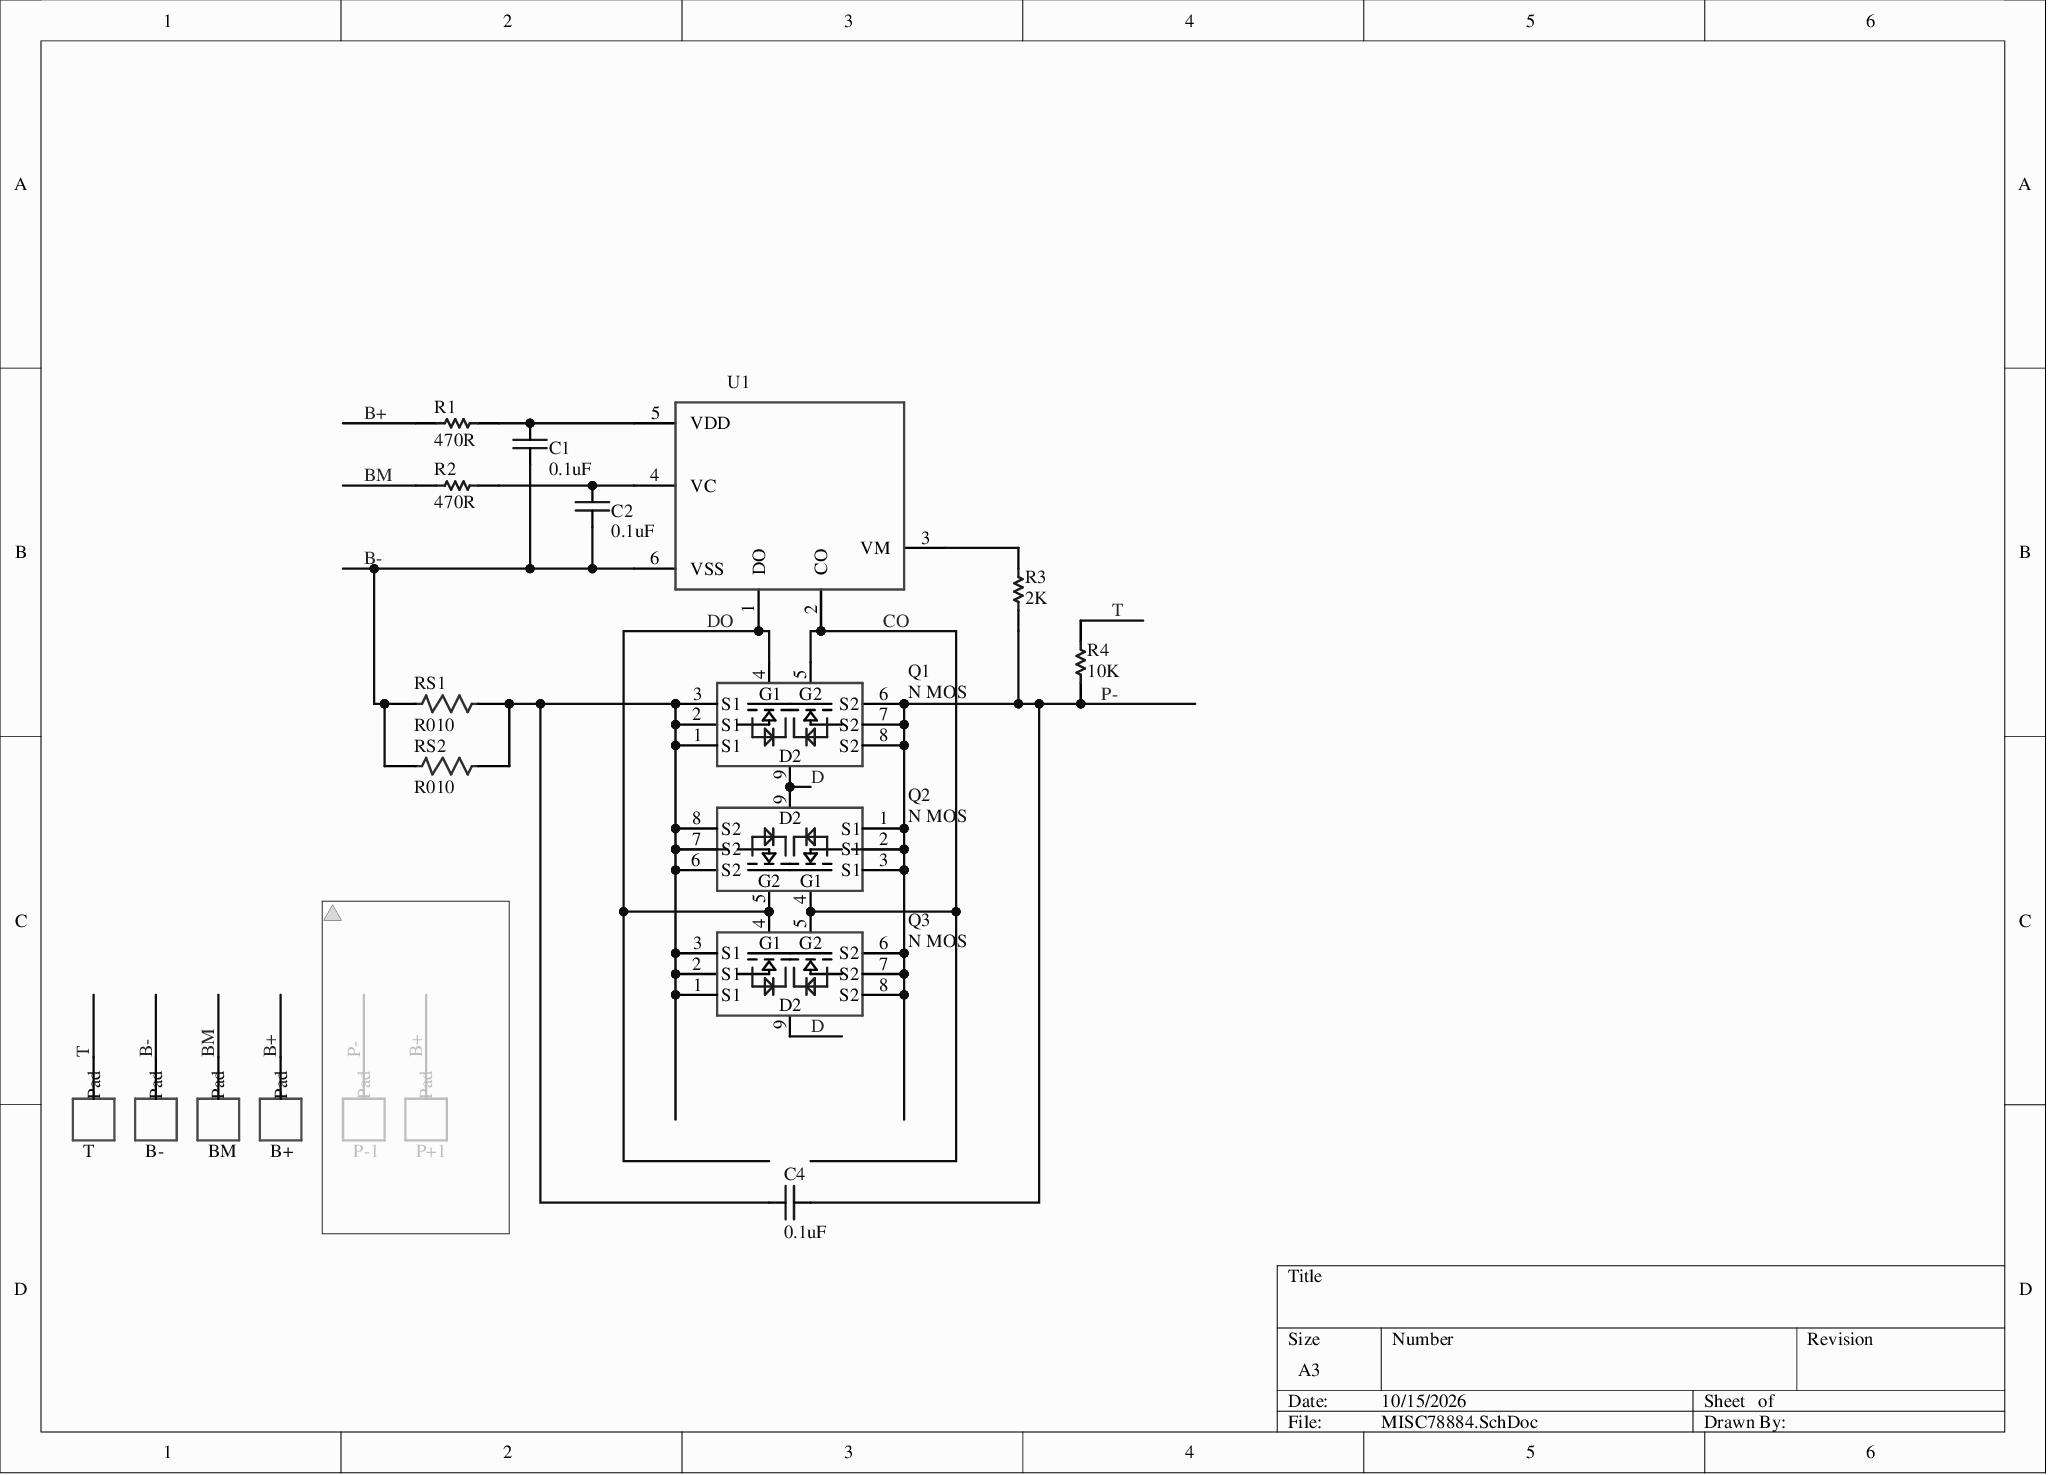
[diagram p0: MISC78884.SchDoc]
# Altium project MISC78884.PrjPcb
1 sheet, 19 parts. Net scope: global (net labels, ports and power ports of the same name join across sheets).
Board file: MISC78884.PcbDoc

## Sheet MISC78884.SchDoc
size 250 x 180 mm; SheetNumber: 1; SheetTotal: 1

### Parts
B+  Pad  [Pad10X8mm]
B-  Pad  [Pad10X8mm]
BM  Pad  [Pad10X8mm]
C1  0.1uF  [C0402A]
C2  0.1uF  [C0402A]
C4  0.1uF  [C0402A]
P+1  Pad  [Pad10X8mm]  (masked out: inside a compile mask, not in the netlist)
P-1  Pad  [Pad10X8mm]  (masked out: inside a compile mask, not in the netlist)
Q1  N MOS  [DFN3*3-L8(2N)]
Q2  N MOS  [DFN3*3-L8(2N)]
Q3  N MOS  [DFN3*3-L8(2N)]
R1  470R  [R0402A]
R2  470R  [R0402A]
R3  2K  [R0402A]
R4  10K  [R0402A]
RS1  R010  [R2512L]
RS2  R010  [R2512L]
T  Pad  [Pad10X8mm]
U1  (no value)  [SOT23-6A]

### Nets
B+: B+.1 R1.1
B-: B-.1 C1.1 C2.1 RS1.1 RS2.1 U1.6(VSS)
BM: BM.1 R2.1
CO: Q1.5(G2) Q2.4(G1) Q3.5(G2) U1.2(CO)
D: Q1.9(D2) Q2.9(D2) Q3.9(D2)
DO: Q1.4(G1) Q2.5(G2) Q3.4(G1) U1.1(DO)
P-: C4.1 Q1.6(S2) Q1.7(S2) Q1.8(S2) Q2.1(S1) Q2.2(S1) Q2.3(S1) Q3.6(S2) Q3.7(S2) Q3.8(S2) R3.1 R4.1
T: R4.2 T.1
NetC1_2: C1.2 R1.2 U1.5(VDD)
NetC2_2: C2.2 R2.2 U1.4(VC)
NetC4_2: C4.2 Q1.1(S1) Q1.2(S1) Q1.3(S1) Q2.6(S2) Q2.7(S2) Q2.8(S2) Q3.1(S1) Q3.2(S1) Q3.3(S1) RS1.2 RS2.2
NetR3_2: R3.2 U1.3(VM)

### Library data of the parts
B+ B- BM P+1 P-1 T = Pad: Connection pad (non-through-hole)
C1 C2 C4 = CAP: SMD capacitor
Q1-Q3 = 2N MOS: SMD MOS-TSSOP-8
R1-R4 = RES: SMD resistor
RS1 RS2 = RES2: SMD alloy resistor
U1 = S-8252